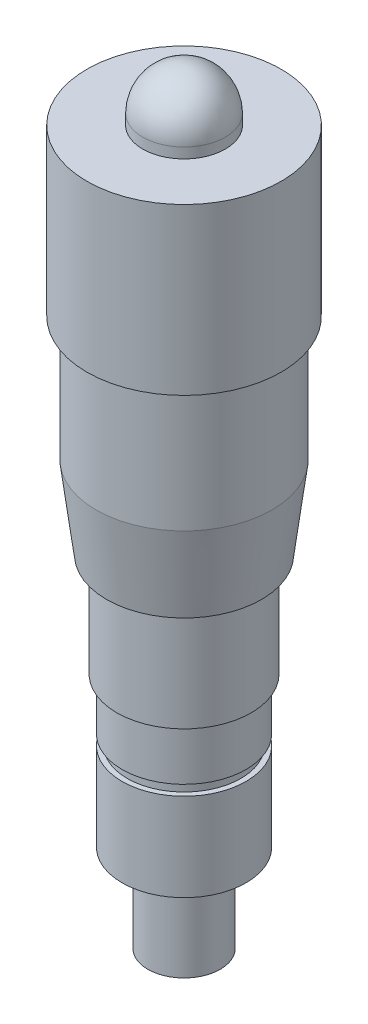
from build123d import *

# Parameters (mm, degrees)
SKETCH1_R           = 1.75
BOSS_EXTRUDE1_DEPTH = 4.25
SKETCH2_R           = 3
BOSS_EXTRUDE2_DEPTH = 4.25
SKETCH3_R           = 2.75
BOSS_EXTRUDE3_DEPTH = 0.5
SKETCH4_R           = 3
BOSS_EXTRUDE4_DEPTH = 2.5
SKETCH5_R           = 3.25
BOSS_EXTRUDE5_DEPTH = 5
SKETCH6_R           = 4.25
BOSS_EXTRUDE6_DEPTH = 10
CHAMFER1_SIZE       = 0.5
CHAMFER1_SIZE2      = 4
SKETCH7_R           = 4.7
BOSS_EXTRUDE7_DEPTH = 8
SKETCH8_R           = 2
BOSS_EXTRUDE8_DEPTH = 2.5
FILLET1_R           = 2


with BuildPart() as part:
    # Sketch1 → Boss-Extrude1 (new body)
    with BuildSketch(Plane(origin=(0, 0, 0), x_dir=(1, 0, 0), z_dir=(0, 1, 0))):
        with Locations(Location((0, 0, 0), (0, 0, 270))):
            Circle(SKETCH1_R)
    extrude(amount=BOSS_EXTRUDE1_DEPTH)

    # Sketch2 → Boss-Extrude2 (add)
    with BuildSketch(Plane(origin=(0, 4.25, 0), x_dir=(1, 0, 0), z_dir=(0, 1, 0))):
        with Locations(Location((0, 0, 0), (0, 0, 270))):
            Circle(SKETCH2_R)
    extrude(amount=BOSS_EXTRUDE2_DEPTH)

    # Sketch3 → Boss-Extrude3 (add)
    with BuildSketch(Plane(origin=(0, 8.5, 0), x_dir=(1, 0, 0), z_dir=(0, 1, 0))):
        with Locations(Location((0, 0, 0), (0, 0, 270))):
            Circle(SKETCH3_R)
    extrude(amount=BOSS_EXTRUDE3_DEPTH)

    # Sketch4 → Boss-Extrude4 (add)
    with BuildSketch(Plane(origin=(0, 9, 0), x_dir=(1, 0, 0), z_dir=(0, 1, 0))):
        with Locations(Location((0, 0, 0), (0, 0, 270))):
            Circle(SKETCH4_R)
    extrude(amount=BOSS_EXTRUDE4_DEPTH)

    # Sketch5 → Boss-Extrude5 (add)
    with BuildSketch(Plane(origin=(0, 11.5, 0), x_dir=(1, 0, 0), z_dir=(0, 1, 0))):
        with Locations(Location((0, 0, 0), (0, 0, 270))):
            Circle(SKETCH5_R)
    extrude(amount=BOSS_EXTRUDE5_DEPTH)

    # Sketch6 → Boss-Extrude6 (add)
    with BuildSketch(Plane(origin=(0, 16.5, 0), x_dir=(1, 0, 0), z_dir=(0, 1, 0))):
        with Locations(Location((0, 0, 0), (0, 0, 270))):
            Circle(SKETCH6_R)
    extrude(amount=BOSS_EXTRUDE6_DEPTH)

    # Chamfer1
    chamfer1_edges = [part.edges().sort_by_distance(p)[0] for p in [
        (0, 16.5, -4.25),
    ]]
    chamfer1_side = [part.faces().sort_by_distance(p)[0] for p in [
        (0, 16.5, -4.129791847),
    ]]
    chamfer(chamfer1_edges, length=CHAMFER1_SIZE, length2=CHAMFER1_SIZE2, reference=chamfer1_side[0])

    # Sketch7 → Boss-Extrude7 (add)
    with BuildSketch(Plane(origin=(0, 26.5, 0), x_dir=(1, 0, 0), z_dir=(0, 1, 0))):
        with Locations(Location((0, 0, 0), (0, 0, 270))):
            Circle(SKETCH7_R)
    extrude(amount=BOSS_EXTRUDE7_DEPTH)

    # Sketch8 → Boss-Extrude8 (add)
    with BuildSketch(Plane(origin=(0, 34.5, 0), x_dir=(1, 0, 0), z_dir=(0, 1, 0))):
        with Locations(Location((0, 0, 0), (0, 0, 270))):
            Circle(SKETCH8_R)
    extrude(amount=BOSS_EXTRUDE8_DEPTH)

    # Fillet1
    fillet1_edges = [part.edges().sort_by_distance(p)[0] for p in [
        (0, 37, -2),
    ]]
    fillet(fillet1_edges, radius=FILLET1_R)


solid = part.part
